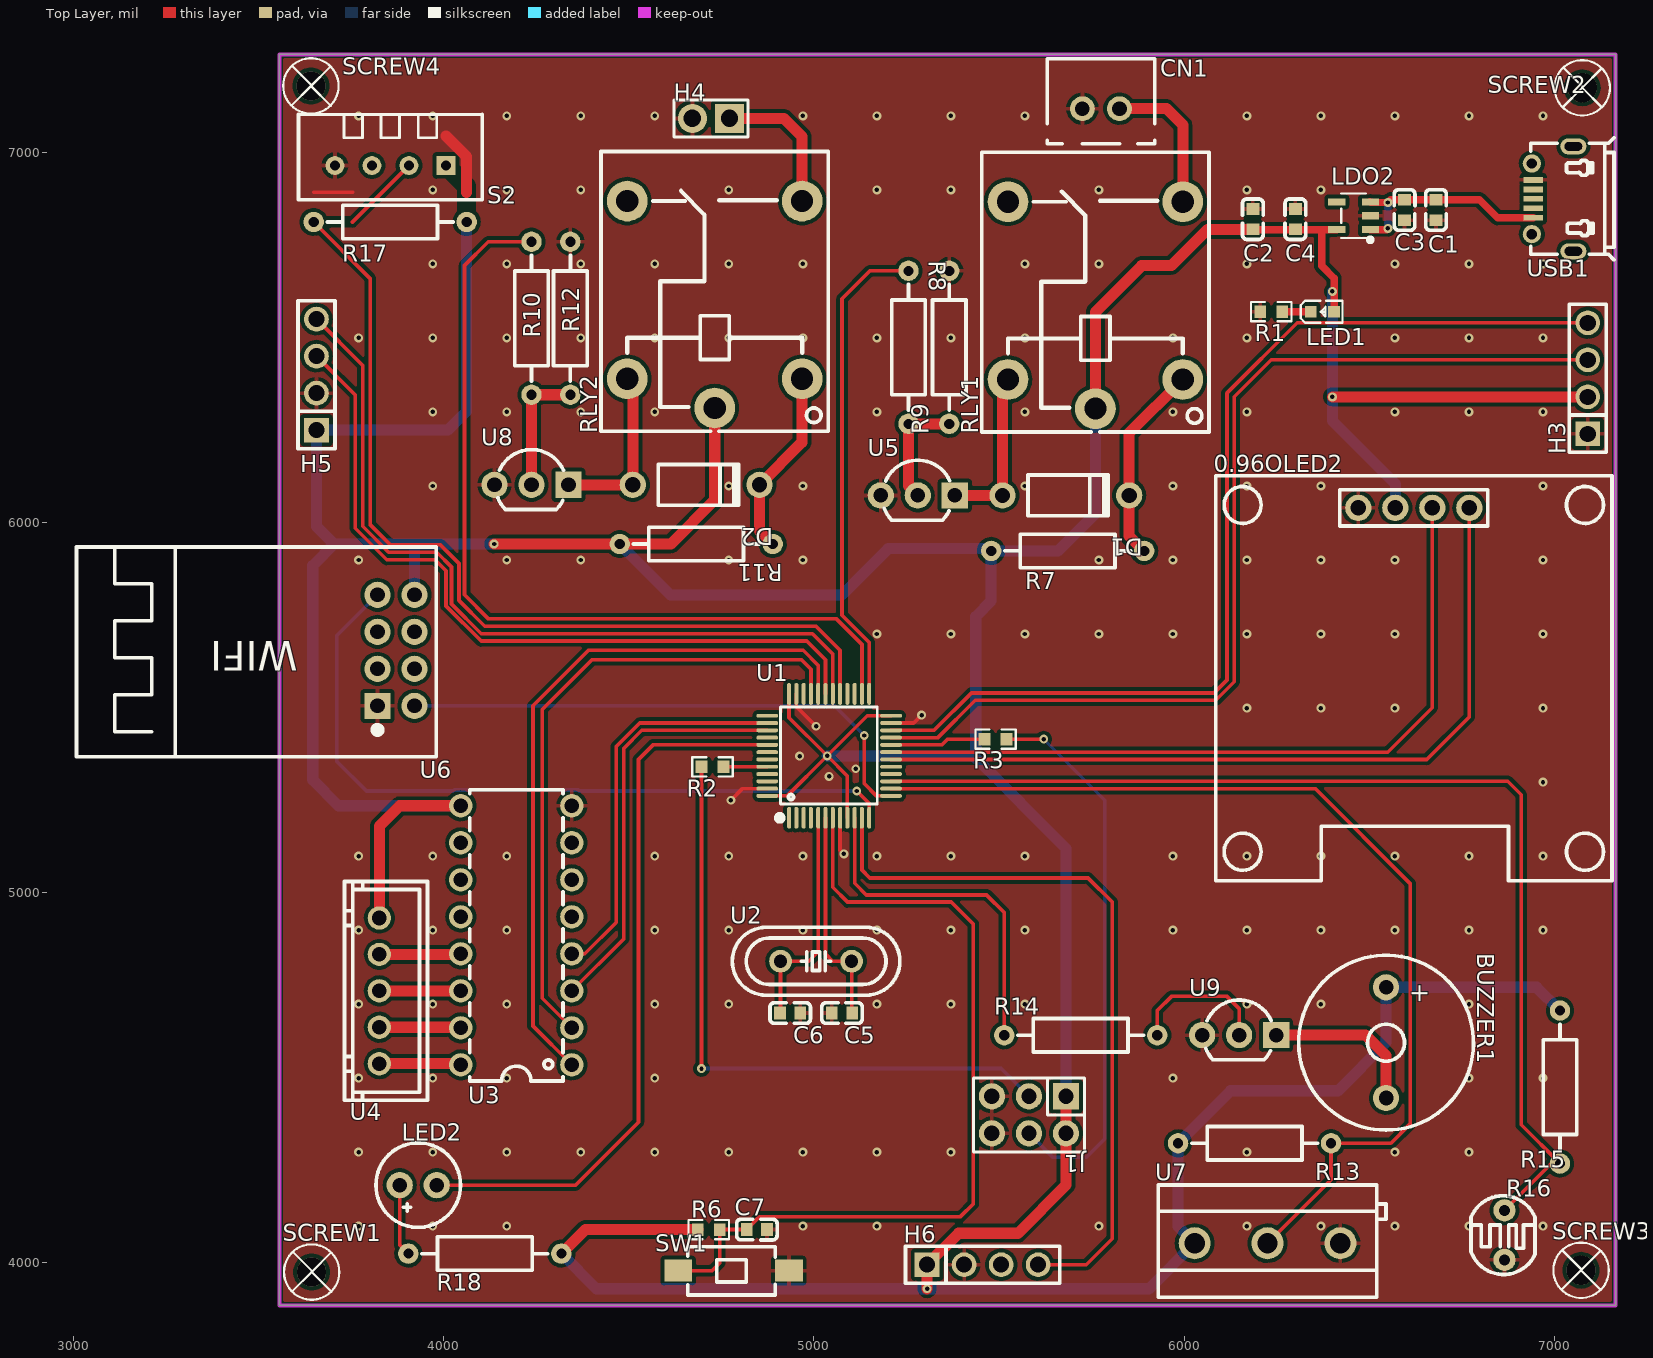
[diagram p0: Top Layer view]
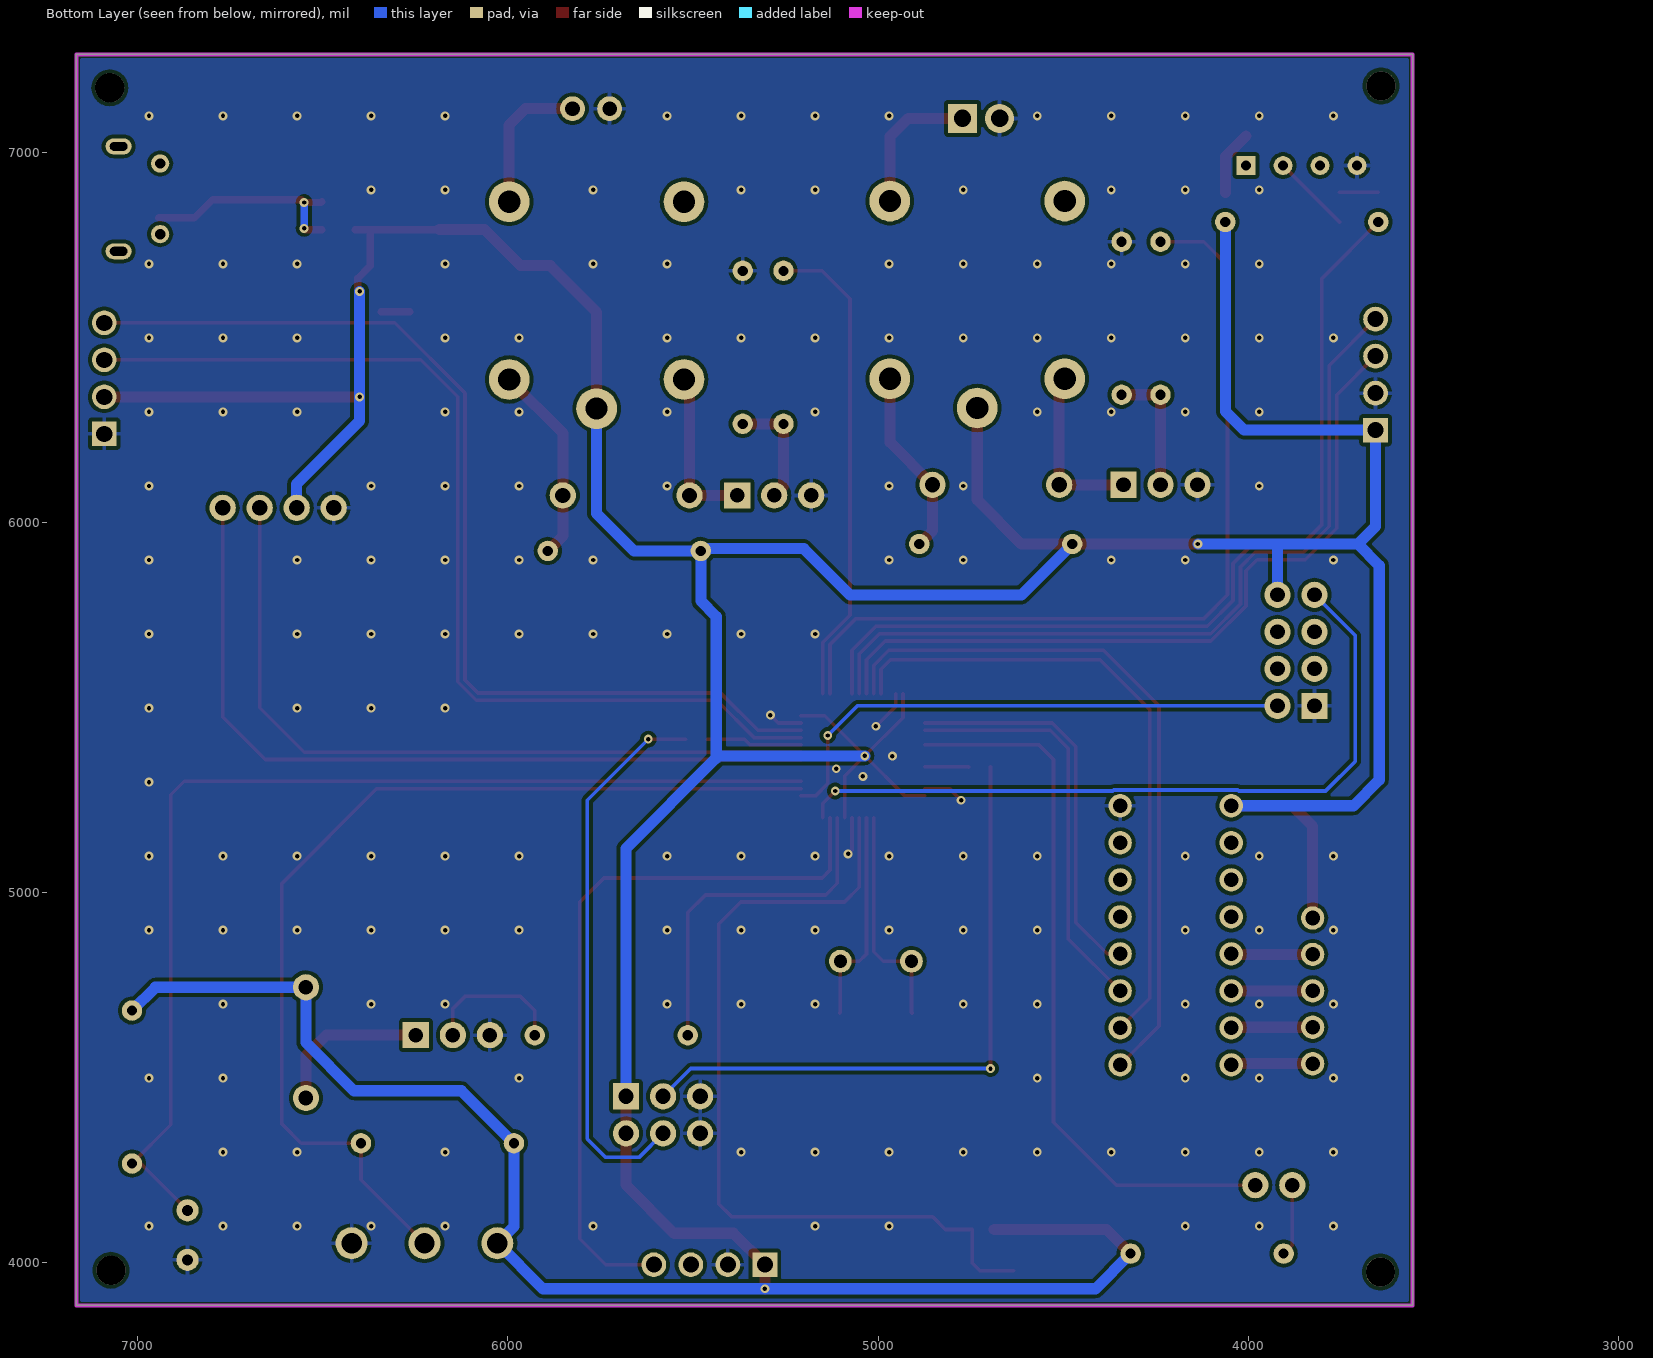
[diagram p1: Bottom Layer view, seen from below]
# Altium PCB MISC51317.pcbdoc
Units mil, origin at the board's own origin, x right, y up, seen from the top; angles counter-clockwise.
Board outline 3610 x 3380 mil, 2 copper layers (Top Layer, Bottom Layer), stack 62.206 mil thick; 54 components, 60 nets, 207 pads, 183 vias.

## Layer stack, top to bottom
Top Solder Mask Layer: solder mask 0.394, Dk 3.3
Top Layer: signal copper 1.379
Dielectric1: surface 59.449, FR4, Dk 4.5
Bottom Layer: signal copper 1.378
Bottom Solder Mask Layer: solder mask 0.394, Dk 3.3

## Board outline
3555.75,7265 3555.75,3885 7165.75,3885 7165.75,7265

## Design rules (kind name [scope] priority, off if disabled: settings)
BoardOutlineClearance copperThickness2oz_1 [All] p2 off: genericclearance=7.99 ignorepadtopadclearanceinfootprint=FALSE except(0: Arc-SplitContinuation Track-SplitContinuation SMDPad-SplitContinuation THPad-SplitContinuation Via-SplitContinuation Fill-SplitContinuation Region-SplitContinuation Poly-SplitContinuation Text-SplitContinuation Hole-SplitContinuation; 5.98: Arc-CutoutEdge SMDPad-CutoutEdge THPad-CutoutEdge Via-CutoutEdge Fill-CutoutEdge Region-CutoutEdge Text-CutoutEdge; 6.93: Hole-OutlineEdge Hole-CutoutEdge; 10: Poly-OutlineEdge Poly-CutoutEdge; 11.81: Arc-OutlineEdge Track-OutlineEdge SMDPad-OutlineEdge THPad-OutlineEdge Via-OutlineEdge Fill-OutlineEdge Region-OutlineEdge Text-OutlineEdge Track-CutoutEdge)
BoardOutlineClearance Plane_innerPlane_1 [All] p4 off: genericclearance=4.02 ignorepadtopadclearanceinfootprint=FALSE except(0: Arc-SplitContinuation Track-SplitContinuation SMDPad-SplitContinuation THPad-SplitContinuation Via-SplitContinuation Fill-SplitContinuation Region-SplitContinuation Poly-SplitContinuation Text-SplitContinuation Hole-SplitContinuation; 6: SMDPad-CutoutEdge THPad-CutoutEdge Via-CutoutEdge Fill-CutoutEdge Region-CutoutEdge Text-CutoutEdge; 6.93: Hole-OutlineEdge Hole-CutoutEdge; 10: Poly-OutlineEdge Poly-CutoutEdge; 11.8: Arc-OutlineEdge Track-OutlineEdge SMDPad-OutlineEdge THPad-OutlineEdge Via-OutlineEdge Fill-OutlineEdge Region-OutlineEdge Text-OutlineEdge; 11.81: Arc-CutoutEdge Track-CutoutEdge)
BoardOutlineClearance Copper_copperRegion_1 [All] p6 off: genericclearance=4.02 ignorepadtopadclearanceinfootprint=FALSE except(0: Arc-SplitContinuation Track-SplitContinuation SMDPad-SplitContinuation THPad-SplitContinuation Via-SplitContinuation Fill-SplitContinuation Region-SplitContinuation Poly-SplitContinuation Text-SplitContinuation Hole-SplitContinuation; 6: SMDPad-CutoutEdge THPad-CutoutEdge Via-CutoutEdge Fill-CutoutEdge Region-CutoutEdge Text-CutoutEdge; 6.93: Hole-OutlineEdge Hole-CutoutEdge; 10: Poly-OutlineEdge Poly-CutoutEdge; 11.8: Arc-OutlineEdge Track-OutlineEdge SMDPad-OutlineEdge THPad-OutlineEdge Via-OutlineEdge Fill-OutlineEdge Region-OutlineEdge Text-OutlineEdge; 11.81: Arc-CutoutEdge Track-CutoutEdge)
BoardOutlineClearance copperThickness1oz_1 [All] p8: genericclearance=4.02 ignorepadtopadclearanceinfootprint=FALSE except(0: Arc-SplitContinuation Track-SplitContinuation SMDPad-SplitContinuation THPad-SplitContinuation Via-SplitContinuation Fill-SplitContinuation Region-SplitContinuation Poly-SplitContinuation Text-SplitContinuation Hole-SplitContinuation; 6: SMDPad-CutoutEdge THPad-CutoutEdge Via-CutoutEdge Fill-CutoutEdge Region-CutoutEdge Text-CutoutEdge; 6.93: Hole-OutlineEdge Hole-CutoutEdge; 10: Poly-OutlineEdge Poly-CutoutEdge; 11.8: Arc-OutlineEdge Track-OutlineEdge SMDPad-OutlineEdge THPad-OutlineEdge Via-OutlineEdge Fill-OutlineEdge Region-OutlineEdge Text-OutlineEdge; 11.81: Arc-CutoutEdge Track-CutoutEdge)
Clearance copperThickness2oz [All] p1 off: gap=7.99 ignorepadtopadclearanceinfootprint=FALSE except(5.98: SMDPad-Track SMDPad-SMDPad THPad-Track SMDPad-THPad THPad-THPad Track-Via SMDPad-Via THPad-Via Via-Via Fill-Track Region-Track Fill-SMDPad Region-SMDPad Fill-THPad Region-THPad Fill-Via Region-Via Fill-Fill Fill-Region Region-Region Arc-Track Arc-SMDPad Arc-THPad Arc-Via Fill-Arc Region-Arc Arc-Arc Text-Track SMDPad-Text Text-THPad Text-Via Fill-Text Region-Text Arc-Text Text-Text; 6.93: Hole-Track Hole-SMDPad Hole-THPad Hole-Via Fill-Hole Region-Hole Hole-Arc Hole-Text; 10: Poly-Track Poly-SMDPad Poly-THPad Poly-Via Poly-Fill Poly-Region Poly-Poly Poly-Arc Poly-Text Poly-Hole)
Clearance Plane_innerPlane [All] p3 off: gap=4.02 ignorepadtopadclearanceinfootprint=FALSE except(5.98: SMDPad-Track SMDPad-SMDPad THPad-Track SMDPad-THPad THPad-THPad Track-Via SMDPad-Via THPad-Via Via-Via Fill-Track Region-Track Fill-SMDPad Region-SMDPad Fill-THPad Region-THPad Fill-Via Region-Via Fill-Fill Fill-Region Region-Region; 6: Arc-Track Arc-SMDPad Arc-THPad Arc-Via Fill-Arc Region-Arc Arc-Arc Text-Track SMDPad-Text Text-THPad Text-Via Fill-Text Region-Text Arc-Text Text-Text; 6.93: Hole-Track Hole-SMDPad Hole-THPad Hole-Via Fill-Hole Region-Hole Hole-Arc Hole-Text; 10: Poly-Track Poly-SMDPad Poly-THPad Poly-Via Poly-Fill Poly-Region Poly-Poly Poly-Arc Poly-Text Poly-Hole)
Clearance Copper_copperRegion [All] p5 off: gap=4.02 ignorepadtopadclearanceinfootprint=FALSE except(5.98: SMDPad-Track SMDPad-SMDPad THPad-Track SMDPad-THPad THPad-THPad Track-Via SMDPad-Via THPad-Via Via-Via Fill-Track Region-Track Fill-SMDPad Region-SMDPad Fill-THPad Region-THPad Fill-Via Region-Via Fill-Fill Fill-Region Region-Region; 6: Arc-Track Arc-SMDPad Arc-THPad Arc-Via Fill-Arc Region-Arc Arc-Arc Text-Track SMDPad-Text Text-THPad Text-Via Fill-Text Region-Text Arc-Text Text-Text; 6.93: Hole-Track Hole-SMDPad Hole-THPad Hole-Via Fill-Hole Region-Hole Hole-Arc Hole-Text; 10: Poly-Track Poly-SMDPad Poly-THPad Poly-Via Poly-Fill Poly-Region Poly-Poly Poly-Arc Poly-Text Poly-Hole)
Clearance copperThickness1oz [All] p7: gap=4.02 ignorepadtopadclearanceinfootprint=FALSE except(5.98: SMDPad-Track SMDPad-SMDPad THPad-Track SMDPad-THPad THPad-THPad Track-Via SMDPad-Via THPad-Via Via-Via Fill-Track Region-Track Fill-SMDPad Region-SMDPad Fill-THPad Region-THPad Fill-Via Region-Via Fill-Fill Fill-Region Region-Region; 6: Arc-Track Arc-SMDPad Arc-THPad Arc-Via Fill-Arc Region-Arc Arc-Arc Text-Track SMDPad-Text Text-THPad Text-Via Fill-Text Region-Text Arc-Text Text-Text; 6.93: Hole-Track Hole-SMDPad Hole-THPad Hole-Via Fill-Hole Region-Hole Hole-Arc Hole-Text; 10: Poly-Track Poly-SMDPad Poly-THPad Poly-Via Poly-Fill Poly-Region Poly-Poly Poly-Arc Poly-Text Poly-Hole)
DiffPairsRouting differentialPair [All] p1: maxlimit=6 minlimit=6 mostfreqgap=6 toplayer_minwidth=5 toplayer_prefwidth=10 toplayer_maxwidth=100 toplayer_mingap=6 toplayer_prefgap=6 toplayer_maxgap=6 bottomlayer_minwidth=5 bottomlayer_prefwidth=10 bottomlayer_maxwidth=100 bottomlayer_mingap=6 bottomlayer_prefgap=6 bottomlayer_maxgap=6 maxuncoupledlength=10
HoleToHoleClearance otherClearance [All] p1: gap=11.81 allowstackedmicrovias=TRUE
Length netLength [All] p1: minlimit=0 maxlimit=0
PasteMaskExpansion pasteMaskExpansion [All] p1: expansion=0
PlaneConnect innerPlane [All] p1: planeconnectstyle=Relief reliefexpansion=20 reliefentries=4 reliefconductorwidth=10 reliefairgap=10
PolygonConnect copperRegion [All] p1: connectstyle=Relief reliefconductorwidth=10 reliefentries=4 polygonreliefangle="90 Angle" airgapwidth=10 via.connectstyle=Relief via.reliefconductorwidth=10 via.reliefentries=4 via.polygonreliefangle="90 Angle" via.airgapwidth=10
RoutingVias viaSize [All] p1: holewidth=12.01 width=24.02 viastyle="Through Hole" minholewidth=11.81 minwidth=19.68 maxholewidth=248.03 maxwidth=393.7
SolderMaskExpansion solderMaskExpansion [IsVia] p1: expansion=-1000 istentingtop=TRUE
SolderMaskExpansion solderMaskExpansion [All] p2: expansion=2 istentingtop=FALSE
Width copperThickness2oz_2 [All] p1 off: maxlimit=100 minlimit=8 preferedwidth=10
Width copperThickness1oz_2 [All] p2: maxlimit=100 minlimit=5 preferedwidth=10

## Components (designator, comment, footprint, x,y, rotation, side; value= is the part's Value field where it differs from the comment)
0.96OLED2 "" oled-th_l27.8-w27.2-p2.54_c9900033791 6620.75,6040 r0 top
BUZZER1 "2.3kHz" BUZ-TH_BD12.0-P7.60-D0.6-FD 6545.75,4595 r270 top
C1 "0.1UF" C0603 6680.75,6845 r90 top
C2 "0.1UF" C0603 6185.75,6820 r270 top
C3 "1uF" C0603 6595.75,6845 r90 top
C4 "1uF" C0603 6300.75,6820 r270 top
C5 "18pF" C0603 5075.75,4675 r180 top
C6 "18pF" C0603 4935.75,4675 r180 top
C7 "0.1UF" C0603 4845.75,4090 r0 top
CN1 "风扇" CONN-TH_B2B-XH-A-LF-SN 5775.47,7118.67 r0 top
D1 "1N4007" DO-41_BD2.4-L4.7-P8.70-D0.8-RD 5680.47,6073.67 r180 top
D2 "1N4007" DO-41_BD2.4-L4.7-P8.70-D0.8-RD 4681.77,6102.3 r180 top
H3 "JW01" HDR-TH_4P-P2.54-V-M 7090.75,6390 r90 top
H4 "水泵" HDR-TH_2P-P2.54-V-M 4721.77,7092.3 r180 top
H5 "串口" HDR-TH_4P-P2.54-V-M 3655.75,6400 r90 top
H6 "YL-69" HDR-TH_4P-P2.54-V-F 5455.75,3995 r0 top
J1 "2.54-2*3P针" HDR-TH_6P-P2.54-V-M-R2-C3-S2.54-1 5580.75,4400 r180 top
LDO2 "ME6211C33M5G-N" SOT-23-5_L3.0-W1.7-P0.95-LS2.8-BL 6458.12,6829.37 r90 top
LED1 "" LED_0603 6375.75,6570 r0 top
LED2 "" LED-TH_BD5.9-P2.54-RD 3930.75,4210 r180 top
R1 "1kΩ" R0603 6235.75,6570 r180 top
R2 "10kΩ" R0603 4725.75,5340 r180 top
R3 "10kΩ" R0603 5490.75,5415 r180 top
R6 "10kΩ" R0603 4715.75,4090 r180 top
R7 "20Ω" RES-TH_BD2.3-L6.5-P10.50-D0.5 5685.47,5923.67 r180 top
R8 "2kΩ" RES-TH_BD2.3-L6.5-P10.50-D0.5 5255.47,6473.67 r270 top
R9 "20kΩ" RES-TH_BD2.3-L6.5-P10.50-D0.5 5365.47,6473.67 r90 top
R10 "2kΩ" RES-TH_BD2.3-L6.5-P10.50-D0.5 4236.77,6552.3 r270 top
R11 "20Ω" RES-TH_BD2.3-L6.5-P10.50-D0.5 4681.77,5942.3 r180 top
R12 "20kΩ" RES-TH_BD2.3-L6.5-P10.50-D0.5 4341.77,6552.3 r90 top
R13 "4.7kΩ" RES-TH_BD2.3-L6.5-P10.50-D0.5 6190.55,4323.06 r180 top
R14 "4.7kΩ" RES-TH_BD2.3-L6.5-P10.50-D0.5 5720.75,4615 r0 top
R15 "10kΩ" RES-TH_BD2.3-L6.5-P10.50-D0.5 7015.75,4475 r90 top
R16 "GL5528(10-20)" RES-TH_L5.1-W4.3-P3.40-D0.5 6865.75,4075 r0 top
R17 "4.7kΩ" RES-TH_BD2.3-L6.5-P10.50-D0.5 3854.9,6812.48 r0 top
R18 "150Ω" RES-TH_BD2.3-L6.5-P10.50-D0.5 4110.75,4025 r0 top
RLY1 "SRD-05VDC-SL-C" RELAY-TH_SRD-XXVDC-XL-C 5760.43,6587.71 r90 top
RLY2 "SRD-05VDC-SL-C" RELAY-TH_SRD-XXVDC-XL-C 4731.8,6589.38 r90 top
S2 "DHT11" SENSOR-TH_DHT11-1 3855.75,6965 r180 top
SCREW1 "" M2螺丝 3642.7,3975.25 r0 top
SCREW2 "" M2螺丝 7075.75,7175 r0 top
SCREW3 "" M2螺丝 7072.7,3979.96 r0 top
SCREW4 "" M2螺丝 3640.75,7180 r0 top
SW1 "KEY-RESET" SW-SMD_L6.0-W3.3-LS8.0 4782.7,3978.99 r0 top
U1 "STM32F103C8T6" LQFP-48_L7.0-W7.0-P0.50-LS9.0-BL 5041.01,5370.01 r0 top
U2 "8M晶振" HC-49S_L11.5-W4.7-P4.88 5005.75,4815 r0 top
U3 "ULN2003A" DIP-16_L20.0-W6.4-P2.54-LS7.6-BL 4195.75,4885 r90 top
U4 "步进电机" CONN-TH_5P-P2.50_ZHOURI_XH-5PA 3825.75,4735 r90 top
U5 "8050" TO-92-3_L4.8-W3.7-P2.54-R 5280.47,6073.67 r0 top
U6 "2.4GHz" WIFIM-TH_8P-L24.7-W14.4-P2.54 3870.75,5655 r180 top
U7 "DS18B20" CONN-TH_3P-P5.00_KF301-5.0-3P 6225.55,4053.06 r0 top
U8 "8050" TO-92-3_L4.8-W3.7-P2.54-R 4236.77,6102.3 r0 top
U9 "8050" TO-92-3_L4.8-W3.7-P2.54-R 6148.78,4615.35 r0 top
USB1 "MICRO-USB-1" MICRO-USB-SMD_C9900008946 6995.75,6875 r90 top

## Footprints (in the part's own frame and the unit in brackets; to place one, negate y for a bottom-side part, rotate by r counter-clockwise, add the part's x,y. Pads: shape width x height; smd on the part's side, far side on the other; paste and mask are expansions set on the pad)
BUZ-TH_BD12.0-P7.60-D0.6-FD [mm]
  round 1.8 hole 1 paste+0 mask+0.051: 1(-3.8,0) 2(3.8,0)
  silkscreen extent -6,-6 6,6
C0603 [mm]
  rect 0.8x0.9 smd: 1(-0.7,0) 2(0.7,0)
  silkscreen extent -1.39,-0.71 1.39,0.71
CONN-TH_3P-P5.00_KF301-5.0-3P [mm]
  round 2.2 hole 1.4: 1(-5,0) 2(0,0) 3(5,0)
  silkscreen extent -7.5,-3.7 8.13,4
CONN-TH_5P-P2.50_ZHOURI_XH-5PA [mm]
  round 1.6 hole 1 paste+0 mask+0.05: 1(-5,0) 2(-2.5,0) 3(0,0) 4(2.5,0) 5(5,0)
  silkscreen extent -7.5,-3.3 7.5,2.4
CONN-TH_B2B-XH-A-LF-SN [mm]
  round 1.7 hole 1: 1(1.27,0) 2(-1.27,0)
  silkscreen extent -3.68,-2.41 3.68,3.43
DIP-16_L20.0-W6.4-P2.54-LS7.6-BL [mm]
  round 1.6 hole 1: 1(-8.89,-3.81) 2(-6.35,-3.81) 3(-3.81,-3.81) 4(-1.27,-3.81) 5(1.27,-3.81) 6(3.81,-3.81) 7(6.35,-3.81) 8(8.89,-3.81) 9(8.89,3.81) 10(6.35,3.81) 11(3.81,3.81) 12(1.27,3.81) 13(-1.27,3.81) 14(-3.81,3.81) 15(-6.35,3.81) 16(-8.89,3.81)
  silkscreen extent -10,-3.2 10,3.2
DO-41_BD2.4-L4.7-P8.70-D0.8-RD [mm]
  round 1.8 hole 1.05: 1(-4.35,0) 2(4.35,0)
  silkscreen extent -2.92,-1.4 2.6,1.4
HC-49S_L11.5-W4.7-P4.88 [mm]
  round 1.56 hole 0.9: 1(-2.44,0) 2(2.44,0)
  silkscreen extent -5.75,-2.33 5.75,2.33
HDR-TH_2P-P2.54-V-M [mm]
  rect 2x2 hole 1.2: 1(-1.27,0)
  round 2 hole 1.2: 2(1.27,0)
  silkscreen extent -2.54,-1.27 2.54,1.27
HDR-TH_4P-P2.54-V-F [mm]
  rect 1.7x1.7 hole 1.1 paste+0 mask+0.051: 1(-3.81,0)
  round 1.7 hole 1.1 paste+0 mask+0.051: 2(-1.27,0) 3(1.27,0) 4(3.81,0)
  silkscreen extent -5.29,-1.27 5.29,1.27
HDR-TH_4P-P2.54-V-M [mm]
  rect 1.7x1.7 hole 1.1: 1(-3.81,0)
  round 1.7 hole 1.1: 2(-1.27,0) 3(1.27,0) 4(3.81,0)
  silkscreen extent -5.08,-1.27 5.08,1.27
HDR-TH_6P-P2.54-V-M-R2-C3-S2.54-1 [mm]
  rect 1.8x1.8 hole 1.05: 1(-2.54,-1.27)
  round 1.8 hole 1.05: 2(-2.54,1.27) 3(0,-1.27) 4(0,1.27) 5(2.54,-1.27) 6(2.54,1.27)
  silkscreen extent -3.81,-2.54 3.81,2.54
LED-TH_BD5.9-P2.54-RD [mm]
  round 1.8 hole 1 paste+0 mask+0.05: 1(-1.27,0) 2(1.27,0)
  silkscreen extent -2.9,-2.9 2.9,2.9
LED_0603 [mil]
  rect 31.5x31.5 smd paste+0 mask+2: 1(-33.5,-0.4) 2(29.5,-0.2)
  silkscreen extent -61,-30 53,30
LQFP-48_L7.0-W7.0-P0.50-LS9.0-BL [mm]
  oval 0.27x1.5 smd paste+0 mask+0.05: 1(-2.75,-4.25) 2(-2.25,-4.25) 3(-1.75,-4.25) 4(-1.25,-4.25) 5(-0.75,-4.25) 6(-0.25,-4.25) 7(0.25,-4.25) 8(0.75,-4.25) 9(1.25,-4.25) 10(1.75,-4.25) 11(2.25,-4.25) 12(2.75,-4.25) 25(2.75,4.25) 26(2.25,4.25) 27(1.75,4.25) 28(1.25,4.25) 29(0.75,4.25) 30(0.25,4.25) 31(-0.25,4.25) 32(-0.75,4.25) 33(-1.25,4.25) 34(-1.75,4.25) 35(-2.25,4.25) 36(-2.75,4.25)
  oval 1.5x0.27 smd paste+0 mask+0.05: 13(4.25,-2.75) 14(4.25,-2.25) 15(4.25,-1.75) 16(4.25,-1.25) 17(4.25,-0.75) 18(4.25,-0.25) 19(4.25,0.25) 20(4.25,0.75) 21(4.25,1.25) 22(4.25,1.75) 23(4.25,2.25) 24(4.25,2.75) 37(-4.25,2.75) 38(-4.25,2.25) 39(-4.25,1.75) 40(-4.25,1.25) 41(-4.25,0.75) 42(-4.25,0.25) 43(-4.25,-0.25) 44(-4.25,-0.75) 45(-4.25,-1.25) 46(-4.25,-1.75) 47(-4.25,-2.25) 48(-4.25,-2.75)
  silkscreen extent -3.59,-4.46 3.3,3.34
M2螺丝 [mm]
  round 2 hole 2: 1(0,0)
  silkscreen extent -1.9,-1.9 1.9,1.9
MICRO-USB-SMD_C9900008946 [mm]
  rect 0.4x1.35 smd paste-100 mask+0.051: 1(-1.3,1.325) 2(-0.65,1.325) 3(0,1.325) 4(0.65,1.325) 5(1.3,1.325)
  oval 1.1x1.8 hole 0.6 slot 1.2 at 90 deg: 6(-3.6,-1.425) 6(3.6,-1.425)
  round 1.25 hole 0.7: 6(-2.425,1.425) 6(2.425,1.425)
  silkscreen extent -4.19,-4.22 4.19,1.5
oled-th_l27.8-w27.2-p2.54_c9900033791 [mm]
  round 1.8 hole 1.05 paste+0 mask+0.05: 1(-3.81,0) 2(-1.27,0) 3(1.27,0) 4(3.81,0)
  silkscreen extent -13.6,-25.6 13.6,2.2
R0603 [mil]
  rect 31.75x34.02 smd paste-3937.01 mask+2: 1(-29.66,0) 2(29.66,0)
  silkscreen extent -55,-26 55,26
RELAY-TH_SRD-XXVDC-XL-C [mil]
  round 110 hole 60: 1(-200.79,-236.22) 2(279.53,-236.2) 3(279.53,236.2) 4(-200.79,236.22) 5(-279.53,0)
  silkscreen extent -342,-307 413,307
RES-TH_BD2.3-L6.5-P10.50-D0.5 [mm]
  round 1.4 hole 0.7 paste+0 mask+0.051: 1(-5.25,0) 2(5.25,0)
  silkscreen extent -4.32,-1.15 4.32,1.15
RES-TH_L5.1-W4.3-P3.40-D0.5 [mil]
  round 60 hole 30: 1(0,66.93) 2(0,-66.93)
  silkscreen extent -91,-106 83,106
SENSOR-TH_DHT11-1 [mil]
  rect 51x51 hole 28: 1(-150,0)
  round 51 hole 28: 2(-50,0) 3(50,0) 4(150,0)
  silkscreen extent -248,-138 248,93
SOT-23-5_L3.0-W1.7-P0.95-LS2.8-BL [mm]
  rect 0.49x1.157 smd: 1(-0.95,-1.154) 2(0,-1.154) 3(0.95,-1.154)
  rect 0.49x1.175 smd: 4(0.95,1.154) 5(-0.95,1.154)
  silkscreen extent -1.8,-1.29 1.53,0.85
SW-SMD_L6.0-W3.3-LS8.0 [mm]
  rect 1.9x1.5 smd: 1(-3.8,0) 2(3.8,0)
  silkscreen extent -3.14,-1.67 2.86,1.63
TO-92-3_L4.8-W3.7-P2.54-R [mm]
  rect 1.8x1.8 hole 1 paste+0 mask+0.051: 1(2.54,0)
  round 1.8 hole 1 paste+0 mask+0.051: 2(0,0) 3(-2.54,0)
  silkscreen extent -2.3,-1.7 2.2,2.41
WIFIM-TH_8P-L24.7-W14.4-P2.54 [mm]
  rect 1.8x1.8 hole 1: 1(1.27,3.81)
  round 1.8 hole 1: 2(1.27,1.27) 3(1.27,-1.27) 4(1.27,-3.81) 5(-1.27,3.81) 6(-1.27,1.27) 7(-1.27,-1.27) 8(-1.27,-3.81)
  silkscreen extent -2.77,-7.11 21.93,7.31

## Via types
v1: diameter 24.02, hole 12, Top Layer to Bottom Layer, 183 vias

## Nets (pads, with @x,y where several pads share a name; then routed paths per layer and width w, separated by ;. In a path a pad name is that pad's centre, name@x,y a point inside that pad or via, vN(x,y) a via of type N, cw(c..) or ccw(c..) an arc to the next point about the centre after c; other vN are vias at no path point)
3V3: 0.96OLED2.2 BUZZER1.1 C2.2 C4.2 H3.2 H5.1 H6.1 J1.1 J1.2 LDO2.5 LED1.2 R6.2 R7.2 R11.2 R13.2 R15.2 R17.2 R18.2 RLY1.5 RLY2.5 S2.1 U1.9 U1.24 U1.36 U1.48 U3.9 U4.5 U6.8 U7.1 | length 16191.1
  Top Layer w10: U1.48 4927.49,5261.74 v1(5035.75,5370) ; U1.36 4932.74,5473.01 v1(5035.75,5370) ; U1.9 5090.22,5315.53 v1(5035.75,5370) ; U1.24 5144.03,5478.28 v1(5035.75,5370)
  Top Layer w20: C2.2 6186.22,6791.97 6371.9,6791.97 ; LED1.2 6405.25,6660.5 6371.9,6693.85 6371.9,6791.97 ; LDO2.5 6371.9,6791.97
  Top Layer w30: U4.5 3825.75,5180 3880.75,5235 U3.9 ; 4005.75,7045 4061.59,6989.16 4061.59,6892.48 ; v1(4135.75,5942.3) R11.2 4613.05,5942.3 4731.8,6061.05 RLY2.5 ; R18.2 4382.44,4090 R6.2 ; v1(5305.75,3930) H6.1 5390.75,4080 5550.75,4080 5680.75,4210 J1.2 J1.1 ; RLY1.5 5760.43,6569.68 5885.75,6695 5965.75,6695 6063.19,6792.44 C2.2 ; v1(6400.75,6340) H3.2
  Bottom Layer w30: U6.8 3920.75,5942.3 ; U3.9 3715.75,5235 3645.75,5305 3645.75,5884.59 3703.45,5942.3 ; R17.2 4061.59,6300.84 4010.75,6250 H5.1 3655.75,5990 3703.45,5942.3 ; v1(4135.75,5942.3) 3920.75,5942.3 ; R18.2 4412.44,3930 v1(5305.75,3930) 5905.64,3930 U7.1 5983.86,4097.9 R13.2 6125.8,4465 6415.75,4465 6545.75,4595 BUZZER1.1 6952.84,4744.6 R15.2 ; R11.2 4612.38,5805 5075.75,5805 5200.75,5930 5472.45,5930 R7.2 ; v1(5035.75,5370) 5430.75,5370 5437.2,5363.55 ; J1.1 5680.75,5120 5437.2,5363.55 ; RLY1.5 5760.43,6024.68 5659.42,5923.67 R7.2 ; v1(6400.75,6625) v1(6400.75,6340) 6400.75,6275 6570.75,6105 0.96OLED2.2 ; 3703.45,5942.3 3920.75,5942.3 ; 5437.2,5363.55 5437.2,5746.45 5478.78,5788.03 R7.2
$1N14: LED1.1 R1.1 | length 77
  Top Layer w20: R1.1 6341.85,6570 LED1.1
$1N19: J1.3 R2.2 | length 1730.7
  Top Layer w10: v1(4696.09,4525) R2.2
  Bottom Layer w10: v1(4696.09,4525) 5505.75,4525 J1.3
$1N20: J1.4 R3.1 | length 1501.3
  Top Layer w10: R3.1 v1(5620.75,5415)
  Bottom Layer w10: J1.4 5645.75,4285 5735.75,4285 5785.75,4335 5785.75,5250 v1(5620.75,5415)
$1N36: U3.13 U4.4 | length 220.7
  Top Layer w30: U4.4 4044.18,4833.43 U3.13
$1N37: U3.14 U4.3 | length 220
  Top Layer w30: U4.3 U3.14
$1N38: U3.15 U4.2 | length 220.7
  Top Layer w30: U4.2 4044.17,4636.58 U3.15
$1N39: U3.16 U4.1 | length 221.3
  Top Layer w30: U4.1 4042.6,4538.15 U3.16
$1N100: D1.2 RLY1.4 U5.1 | length 448.2
  Top Layer w30: U5.1 D1.2 5509.21,6371.92 RLY1.4
$1N101: D1.1 R7.1 RLY1.1 | length 540
  Top Layer w30: R7.1 5851.73,5964.1 D1.1 5851.73,6242 RLY1.1
$1N103: R8.2 R9.1 U5.2 | length 313.7
  Top Layer w30: U5.2 5255.47,6098.67 R8.2 R9.1
$1N118: D2.2 RLY2.4 U8.1 | length 466.2
  Top Layer w30: U8.1 D2.2 4510.51,6373.66 RLY2.4
$1N119: D2.1 R11.1 RLY2.1 | length 508.6
  Top Layer w30: R11.1 4853.03,5977.73 D2.1 4968.02,6217.28 RLY2.1
$1N121: R10.2 R12.1 U8.2 | length 348.3
  Top Layer w30: U8.2 R10.2 R12.1
$1N141: H6.3
$1N143: BUZZER1.2 U9.1 | length 434.5
  Top Layer w30: U9.1 6490.4,4615.35 6545.75,4560 BUZZER1.2
$1N144: R14.2 U9.2 | length 389.2
  Top Layer w10: R14.2 5927.44,4681.69 5965.75,4720 6115.75,4720 6148.78,4686.97 U9.2
$1N155: LED2.2 R18.1 | length 194.7
  Top Layer w10: LED2.2 3880.75,4048.31 R18.1
+5V: C1.2 C3.2 LDO2.1 LDO2.3 USB1.1 | length 582.6
  Top Layer w20: LDO2.1 6547.72,6791.97 v1(6550.75,6795) ; LDO2.3 6505.31,6865 v1(6550.75,6865) 6558.31,6872.56 C3.2 C1.2 6798.19,6872.56 6846.93,6823.82 USB1.1
  Bottom Layer w20: v1(6550.75,6795) v1(6550.75,6865)
BOOT0: R2.1 U1.44 | length 118.5
  Top Layer w10: R2.1 4755.89,5340.48 U1.44
BOOT1: R3.2 U1.20 | length 259.2
  Top Layer w10: U1.20 5345.29,5399.54 5360.75,5415 R3.2
D+: USB1.3
D-: USB1.2
GND: 0.96OLED2.1 C1.1 C2.1 C3.1 C4.1 C5.2 C6.1 C7.2 CN1.2 H3.1 H4.2 H5.2 H6.2 J1.5 J1.6 LDO2.2 R1.2 R9.2 R12.2 R16.2 S2.4 SW1.2 U1.8 U1.23 U1.35 U1.47 U3.8 U5.3 U6.1 U7.3 U8.3 U9.3 USB1.5 | length 413.6
  Top Layer w10: v1(4775.75,5250) 4807.18,5281.43 U1.47 ; U1.35 4952.43,5503.32 v1(5005.75,5450) ; U1.8 5070.54,5115.21 v1(5080.75,5105) ; U1.23 5269.34,5458.59 v1(5290.75,5480)
  other v1: 3769.85,4099.1 3969.85,4099.1 4169.85,4099.1 4969.85,4099.1 5169.85,4099.1 5769.85,4099.1 6169.85,4099.1 6369.85,4099.1 6569.85,4099.1 6769.85,4099.1 6969.85,4099.1 3769.85,4299.1 3969.85,4299.1 4169.85,4299.1 4369.85,4299.1 4569.85,4299.1 4769.85,4299.1 4969.85,4299.1 5169.85,4299.1 5369.85,4299.1 6169.85,4299.1 6569.85,4299.1 6769.85,4299.1 3769.85,4499.1 3969.85,4499.1 4169.85,4499.1 4569.85,4499.1 5969.85,4499.1 6769.85,4499.1 6969.85,4499.1 3769.85,4699.1 3969.85,4699.1 4169.85,4699.1 4569.85,4699.1 4769.85,4699.1 5169.85,4699.1 5369.85,4699.1 5569.85,4699.1 6169.85,4699.1 6369.85,4699.1 6769.85,4699.1 3769.85,4899.1 3969.85,4899.1 4169.85,4899.1 4569.85,4899.1 4769.85,4899.1 4969.85,4899.1 5169.85,4899.1 5369.85,4899.1 5569.85,4899.1 5969.85,4899.1 6169.85,4899.1 6369.85,4899.1 6569.85,4899.1 6769.85,4899.1 6969.85,4899.1 3769.85,5099.1 3969.85,5099.1 4169.85,5099.1 4569.85,5099.1 4769.85,5099.1 4969.85,5099.1 5169.85,5099.1 5369.85,5099.1 5569.85,5099.1 5969.85,5099.1 6169.85,5099.1 6369.85,5099.1 6569.85,5099.1 6769.85,5099.1 6969.85,5099.1 6969.85,5299.1 5041.01,5314.31 5112.76,5335 4961.19,5369.02 6169.85,5499.1 6369.85,5499.1 6569.85,5499.1 6969.85,5499.1 5169.85,5699.1 5369.85,5699.1 5569.85,5699.1 5769.85,5699.1 5969.85,5699.1 6169.85,5699.1 6369.85,5699.1 6569.85,5699.1 6969.85,5699.1 3769.85,5899.1 4169.85,5899.1 4369.85,5899.1 4769.85,5899.1 4969.85,5899.1 5769.85,5899.1 5969.85,5899.1 6169.85,5899.1 6369.85,5899.1 6569.85,5899.1 6969.85,5899.1 3969.85,6099.1 4769.85,6099.1 4969.85,6099.1 5569.85,6099.1 5969.85,6099.1 6169.85,6099.1 6369.85,6099.1 6969.85,6099.1 3969.85,6299.1 4169.85,6299.1 4369.85,6299.1 4569.85,6299.1 5169.85,6299.1 5569.85,6299.1 5969.85,6299.1 6169.85,6299.1 6569.85,6299.1 6769.85,6299.1 6969.85,6299.1 3769.85,6499.1 3969.85,6499.1 4169.85,6499.1 4369.85,6499.1 4569.85,6499.1 4769.85,6499.1 4969.85,6499.1 5169.85,6499.1 5369.85,6499.1 5569.85,6499.1 5969.85,6499.1 6169.85,6499.1 6569.85,6499.1 6769.85,6499.1 6969.85,6499.1 3969.85,6699.1 4169.85,6699.1 4369.85,6699.1 4569.85,6699.1 4769.85,6699.1 4969.85,6699.1 5569.85,6699.1 5769.85,6699.1 6169.85,6699.1 6569.85,6699.1 6769.85,6699.1 6969.85,6699.1 3969.85,6899.1 4169.85,6899.1 4369.85,6899.1 4769.85,6899.1 5169.85,6899.1 5369.85,6899.1 5769.85,6899.1 6169.85,6899.1 6369.85,6899.1 3769.85,7099.1 3969.85,7099.1 4169.85,7099.1 4369.85,7099.1 4569.85,7099.1 4969.85,7099.1 5169.85,7099.1 5369.85,7099.1 5569.85,7099.1 6169.85,7099.1 6369.85,7099.1 6569.85,7099.1 6769.85,7099.1 6969.85,7099.1
OSCIN: C6.2 U1.5 U2.1 | length 615
  Top Layer w10: C6.2 4909.69,4676.5 U2.1 4985.75,4815 5011.48,4840.73 U1.5
OSCOUT: C5.1 U1.6 U2.2 | length 587.5
  Top Layer w10: U1.6 5031.17,4834.58 5050.75,4815 U2.2 5101.81,4676.5 C5.1
PA0: R14.1 U1.10 | length 945.5
  Top Layer w10: U1.10 5109.91,5025.84 5141.53,4994.22 5466.53,4994.22 5514.06,4946.69 R14.1
PA1: H6.4 U1.11 | length 1992.4
  Top Layer w10: U1.11 5129.59,5061.16 5150.75,5040 5740.75,5040 5805.75,4975 5805.75,4065 5735.75,3995 H6.4
PA2: U1.12 U6.4 | length 2022
  Top Layer w10: v1(5115.75,5275) 5149.28,5241.47 U1.12
  Bottom Layer w10: U6.4 3710.75,5695 3710.75,5355 3790.75,5275 4025.67,5275 4028.15,5277.48 4363.35,5277.48 4365.83,5275 v1(5115.75,5275)
PA3: U1.13 U6.5 | length 1464.5
  Top Layer w10: v1(5135.75,5425) 5135.75,5295 5169.01,5261.74 U1.13
  Bottom Layer w10: U6.5 5055.75,5505 v1(5135.75,5425)
PA4: R13.1 U1.14 U7.2 | length 2734.8
  Top Layer w10: U1.14 6354.32,5281.43 6610.75,5025 6610.75,4375 6558.81,4323.06 R13.1 6397.24,4224.75 U7.2
PA5: R15.1 R16.1 U1.15 | length 2959.9
  Top Layer w10: U1.15 6874.64,5301.11 6910.75,5265 6910.75,4373.31 R15.1 6992.13,4268.31 R16.1
PA6: U1.16
PA7: U1.17
PA8: R17.1 S2.2 U1.29 | length 2788.4
  Top Layer w10: R17.1 3800.75,6659.94 3800.75,5995 3855.75,5940 3990.75,5940 4040.75,5890 4040.75,5790 4110.75,5720 5005.75,5720 5070.54,5655.21 U1.29 ; 3648.21,6892.48 3753.23,6892.48 ; 3753.23,6812.48 S2.2
PA9: H5.4 U1.30 | length 2191
  Top Layer w10: H5.4 3780.75,6425 3780.75,5990 3850.75,5920 3980.75,5920 4020.75,5880 4020.75,5780 4100.75,5700 4995.75,5700 5050.85,5644.9 U1.30
PA10: H5.3 U1.31 | length 2074
  Top Layer w10: H5.3 3760.75,6345 3760.75,5985 3845.75,5900 3975.75,5900 4005.75,5870 4005.75,5775 4100.75,5680 4980.75,5680 5031.17,5629.58 U1.31
PA11: U1.32 U3.1 | length 1940.2
  Top Layer w10: U3.1 4240.75,4640 4240.75,5505 4390.75,5655 4970.75,5655 5011.48,5614.27 U1.32
PA12: U1.33 U3.2 | length 1752.5
  Top Layer w10: U3.2 4265.75,4715 4265.75,5495 4400.75,5630 4965.75,5630 4991.8,5603.95 U1.33
PA15: U1.38 U3.4 | length 1064.5
  Top Layer w10: U3.4 4380.75,4835 4465.75,4920 4465.75,5395 4529.34,5458.59 U1.38
PB0: 0.96OLED2.4 U1.18 | length 2175
  Top Layer w10: U1.18 6655.92,5360.17 6770.75,5475 0.96OLED2.4
PB1: 0.96OLED2.3 U1.19 | length 2052.2
  Top Layer w10: U1.19 6550.6,5379.85 6670.75,5500 0.96OLED2.3
PB3: U1.39 U3.3 | length 1121.2
  Top Layer w10: U3.3 4485.75,4875 4485.75,5390 4534.66,5438.91 U1.39
PB4: U1.40
PB5: LED2.1 U1.41 | length 1959.7
  Top Layer w10: LED2.1 4355.75,4210 4525.75,4380 4525.75,5360 4565.29,5399.54 U1.41
PB10: H3.3 U1.21 | length 2756.3
  Top Layer w10: U1.21 5334.97,5419.22 5435.75,5520 6085.75,5520 6135.75,5570 6135.75,6340 6235.75,6440 H3.3
PB11: H3.4 U1.22 | length 2792.5
  Top Layer w10: U1.22 5324.66,5438.91 5425.75,5540 6080.75,5540 6115.75,5575 6115.75,6350 6305.75,6540 H3.4
PB12: R8.1 U1.25 | length 1309.1
  Top Layer w10: U1.25 5149.28,5676.47 5075.75,5750 5075.75,6605 5151.11,6680.36 R8.1
PB13: R10.1 U1.26 | length 2360.6
  Top Layer w10: R10.1 4119.74,6758.99 4055.75,6695 4055.75,5805 4120.75,5740 5060.75,5740 5129.59,5671.16 U1.26
PB14: U1.27
PB15: U1.28
PC13: U1.2
PC14: U1.3
PC15: U1.4
RESET: C7.1 R6.1 SW1.1 U1.7 | length 2289.6
  Top Layer w10: SW1.1 4724.74,3978.99 4745.41,3999.66 R6.1 C7.1 4853.19,4125 5395.75,4125 5430.75,4160 5430.75,4915 5370.75,4975 5090.75,4975 5050.85,5014.9 U1.7
RLY1_NO: CN1.1 RLY1.2 | length 396.5
  Top Layer w30: CN1.1 5952.08,7118.67 5996.63,7074.12 RLY1.2
RLY2_NO: H4.1 RLY2.2 | length 390.6
  Top Layer w30: H4.1 4918.45,7092.3 4968,7042.75 RLY2.2
SWCLK: U1.37
SWDIO: U1.34
VBAT: U1.1
pads on no net: LDO2.4 RLY1.3 RLY2.3 S2.3 SCREW1.1 SCREW2.1 SCREW3.1 SCREW4.1 U1.42 U1.43 U1.45 U1.46 U3.5 U3.6 U3.7 U3.10 U3.11 U3.12 U6.2 U6.3 U6.6 U6.7 USB1.4 USB1.6

## Polygon pours and split planes (outlines as drawn)
GND on Bottom Layer (solid, remove dead copper, pour order 2): 3330.75,7800 3330.75,3000 7695.75,3000 7695.75,7800
GND on Top Layer (solid, remove dead copper, pour order 0): 3350.75,7540 3350.75,3675 7535.75,3675 7535.75,7540

## Keep-outs
Board Outline Layer:
  the board outline again, w10